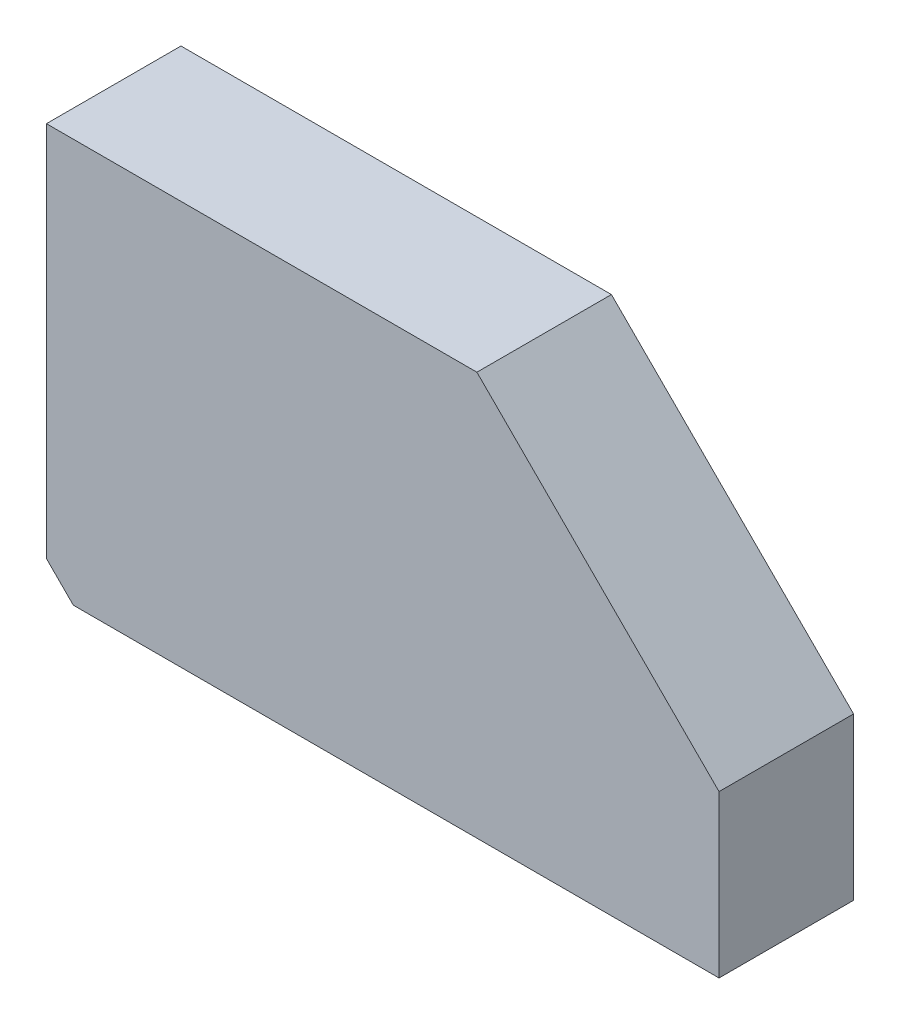
SolidWorks part; units mm, degrees
material "6061-T6 (SS)"
ref_plane "前视基准面" through (0, 0, 0) normal (0, 0, 1) x (1, 0, 0)
ref_plane "上视基准面" through (0, 0, 0) normal (0, 1, 0) x (1, 0, 0)
ref_plane "右视基准面" through (0, 0, 0) normal (1, 0, 0) x (0, 0, -1)
sketch "草图1" plane through (0, 0, 0) normal (0, 0, 1) x (1, 0, 0)
  line L0 (62, -20.9115) -> (12, -20.9115)
  line L2 (12, -20.9115) -> (12, 9.0885)
  line L4 (12, 9.0885) -> (44, 9.0885)
  line L5 (44, 9.0885) -> (62, -8.9115)
  line L6 (62, -8.9115) -> (62, -20.9115)
  dimension "D1" = 30
  dimension "D2" = 50
  dimension "D3" = 12
  dimension "D4" = 45
extrude "凸台-拉伸1" add sketch "草图1" along normal blind 10
chamfer "倒角1" distance 2 angle 45 1 edges at (12, -20.9115, 5)
hole_wizard "M5 螺纹孔1" positions "草图5" profile "草图4" tap size "M5" standard "Iso"
sketch "草图5" plane through (12, 0, 0) normal (-1, 0, 0) x (0, 0, 1)
  line L0 (-15, -20.9115) -> (25, -20.9115) construction
  point P0 (5, -10.9115)
  point P3 (5, 1.0885)
  dimension "D1" = 10
  dimension "D2" = 12
sketch "草图4" plane through (12, -10.9115, 5) normal (0, 1, 0) x (0, 0, 1)
  line L0 (0, 0) -> (0, 15.2618)
  line L1 (0, 15.2618) -> (2.1, 14)
  line L2 (2.1, 14) -> (2.1, 0)
  line L5 (2.1, 0) -> (0, 0)
  line L10 (0, 15.2618) -> (-2.1, 14) construction
  line L11 (0, -6.35) -> (0, 107.95) construction
  dimension "螺纹孔钻头直径" = 4.2
  dimension "螺纹孔钻头深度" = 14
  dimension "导头角度" = 118
cosmetic thread "孔螺蚊线1"
cosmetic thread "孔螺蚊线2"
hole_wizard "M5 螺纹孔2" positions "草图8" profile "草图9" tap size "M5" standard "Iso"
sketch "草图8" plane through (0, -20.9115, 0) normal (0, -1, 0) x (-1, 0, 0)
  point P0 (-30, -5)
  point P3 (-50, -5)
sketch "草图9" plane through (30, -20.9115, 5) normal (1, 0, 0) x (0, 0, -1)
  line L0 (0, 0) -> (0, 15.2618)
  line L1 (0, 15.2618) -> (2.1, 14)
  line L2 (2.1, 14) -> (2.1, 0)
  line L5 (2.1, 0) -> (0, 0)
  line L10 (0, 15.2618) -> (-2.1, 14) construction
  line L11 (0, -6.35) -> (0, 107.95) construction
  dimension "螺纹孔钻头直径" = 4.2
  dimension "螺纹孔钻头深度" = 14
  dimension "导头角度" = 118
cosmetic thread "孔螺蚊线3"
cosmetic thread "孔螺蚊线4"
